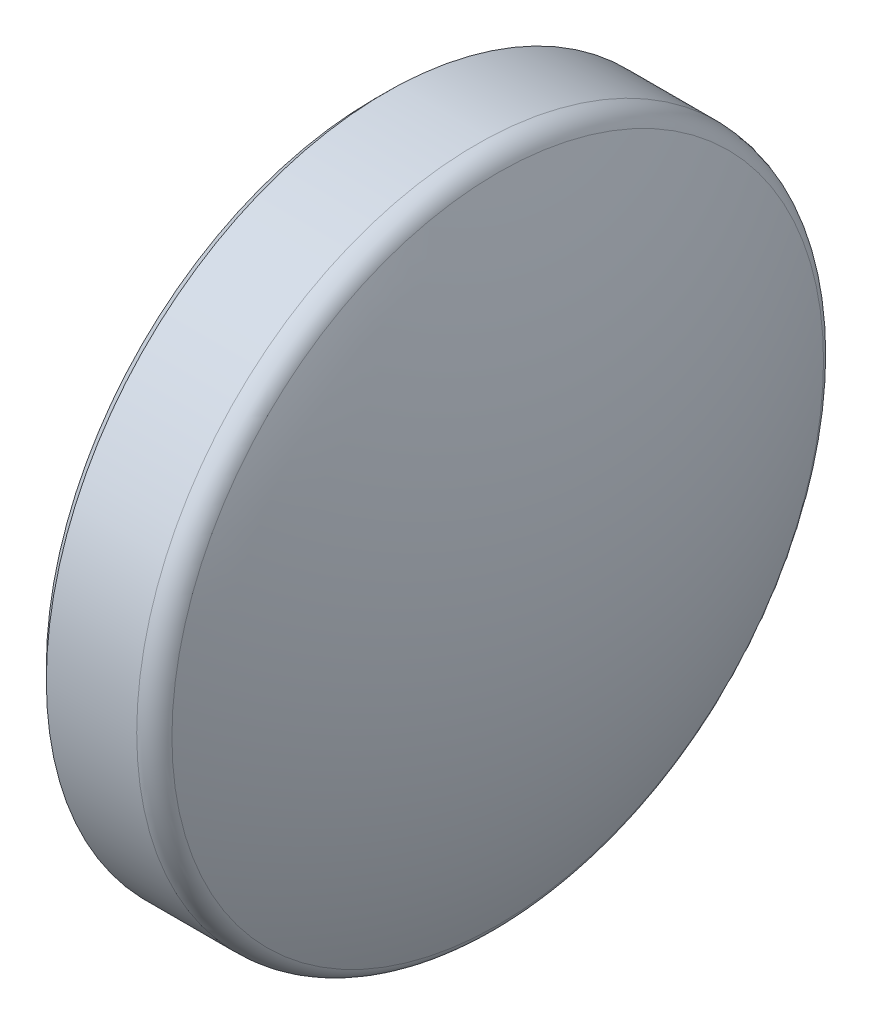
from build123d import *

# Parameters (mm, degrees)
FILLET2_R     = 2
CHAMFER1_SIZE = 1


with BuildPart() as part:
    # Sketch1 → Revolve1 (revolve)
    with BuildSketch(Plane.XY, mode=Mode.PRIVATE) as revolve1_sk:
        with BuildLine():
            Line((0, 0), (10, 0))
            ThreePointArc((10, 0), (14.850570129, 14.140905371), (16.493902741, 29))
            Line((16.493902741, 29), (0, 29))
            Line((0, 29), (0, 0))
        make_face()
    revolve(revolve1_sk.sketch.rotate(Axis((-110.537857647, 29, 0), (1, 0, 0)), 270), axis=Axis((-110.537857647, 29, 0), (1, 0, 0)))

    # Fillet2
    fillet2_edges = [part.edges().sort_by_distance(p)[0] for p in [
        (10, 29, -29),
    ]]
    fillet(fillet2_edges, radius=FILLET2_R)

    # Chamfer1
    chamfer1_edges = [part.edges().sort_by_distance(p)[0] for p in [
        (0, 29, -29),
    ]]
    chamfer(chamfer1_edges, length=CHAMFER1_SIZE)


solid = part.part
